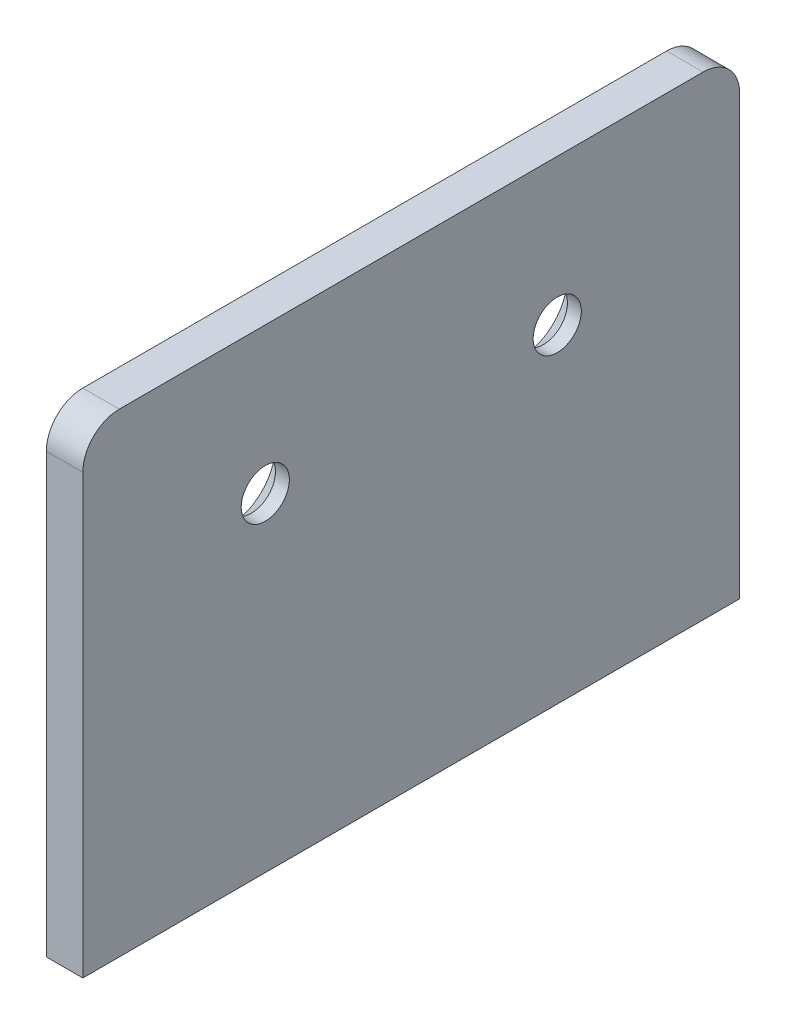
from build123d import *

# Parameters (mm, degrees)
BOSS_EXTRUDE1_DEPTH                         = 5
HOLE_SIZE_BY_HEX_SOCKET_COUNTERSUNK_2_COUNT = 2
HOLE_SIZE_BY_HEX_SOCKET_COUNTERSUNK_2_PITCH = 40


with BuildPart() as part:
    # Sketch1 → Boss-Extrude1 (new body)
    with BuildSketch(Plane(origin=(0, 0, 0), x_dir=(0, 0, -1), z_dir=(1, 0, 0))):
        with BuildLine():
            Line((-45, 60), (-45, 0))
            Line((-45, 0), (45, 0))
            Line((45, 0), (45, 60))
            ThreePointArc((45, 60), (43.535533906, 63.535533906), (40, 65))
            Line((40, 65), (-40, 65))
            ThreePointArc((-40, 65), (-43.535533906, 63.535533906), (-45, 60))
        make_face()
    extrude(amount=BOSS_EXTRUDE1_DEPTH)

    # Sketch2 → Hole size by hex socket countersunk screw type1 (revolve, cut)
    with BuildSketch(Plane(origin=(0, 45, -20), x_dir=(0, 0, 1), z_dir=(0, 1, 0))):
        Polygon((0, 0), (0, 5), (3.3, 5), (3.3, 3.1), (6.4, 0), align=None)
    hole_size_by_hex_socket_countersunk_scre = revolve(axis=Axis((-6.35, 45, -20), (1, 0, 0)), mode=Mode.SUBTRACT)

    # Hole size by hex socket countersunk  2: Hole size by hex socket countersunk screw type1 ×2
    with Locations(*[(0, 0, i * HOLE_SIZE_BY_HEX_SOCKET_COUNTERSUNK_2_PITCH) for i in range(1, HOLE_SIZE_BY_HEX_SOCKET_COUNTERSUNK_2_COUNT)]):
        add(hole_size_by_hex_socket_countersunk_scre, mode=Mode.SUBTRACT)


solid = part.part
